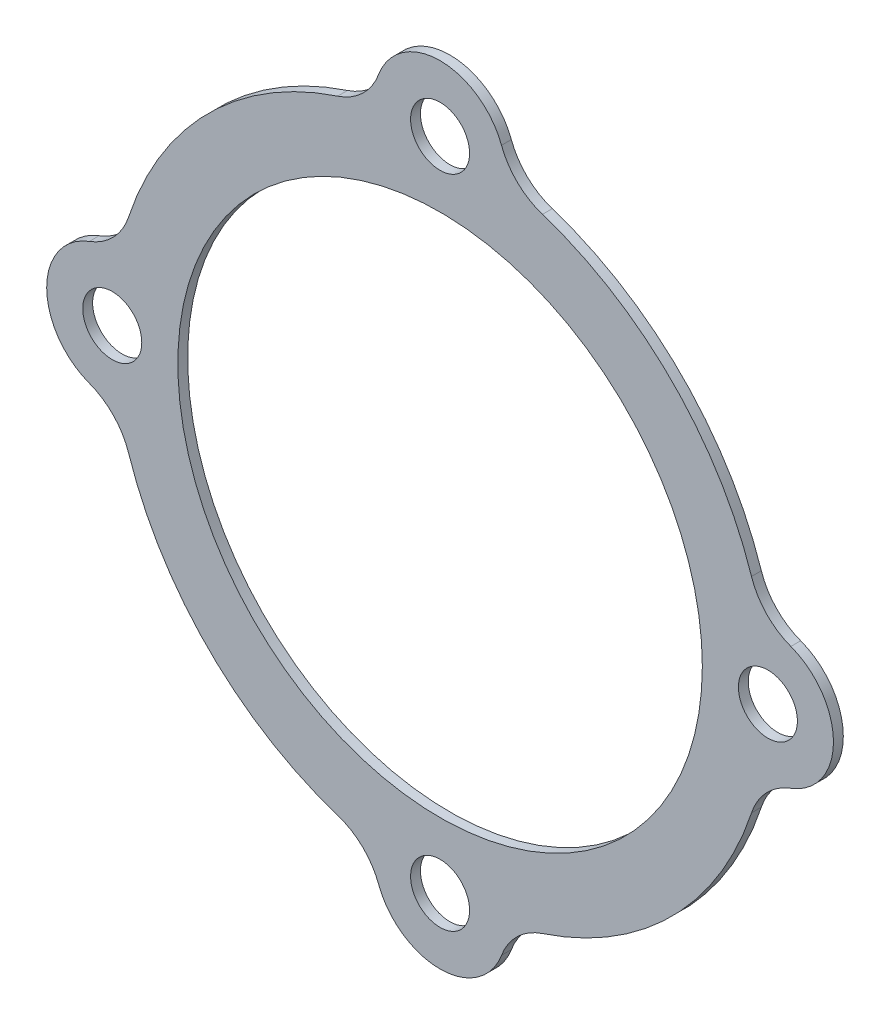
from build123d import *

# Parameters (mm, degrees)
SKETCH_1_R      = 40
SKETCH_1_R_2    = 4.5
EXTRUDE_1_DEPTH = 1.5


with BuildPart() as part:
    # 草图1 → 凸台-拉伸1 (new body)
    with BuildSketch(Plane.XY):
        with BuildLine():
            ThreePointArc((15.612494996, -47.5), (35.355339059, -35.355339059), (47.5, -15.612494996))
            ThreePointArc((47.5, -15.612494996), (49.788897449, -11.806790765), (53.5, -9.367496998))
            ThreePointArc((53.5, -9.367496998), (60, 0), (53.5, 9.367496998))
            ThreePointArc((53.5, 9.367496998), (49.788897449, 11.806790765), (47.5, 15.612494996))
            ThreePointArc((47.5, 15.612494996), (35.355339059, 35.355339059), (15.612494996, 47.5))
            ThreePointArc((15.612494996, 47.5), (11.806790765, 49.788897449), (9.367496998, 53.5))
            ThreePointArc((9.367496998, 53.5), (0, 60), (-9.367496998, 53.5))
            ThreePointArc((-9.367496998, 53.5), (-11.806790765, 49.788897449), (-15.612494996, 47.5))
            ThreePointArc((-15.612494996, 47.5), (-35.355339059, 35.355339059), (-47.5, 15.612494996))
            ThreePointArc((-47.5, 15.612494996), (-49.788897449, 11.806790765), (-53.5, 9.367496998))
            ThreePointArc((-53.5, 9.367496998), (-60, 0), (-53.5, -9.367496998))
            ThreePointArc((-53.5, -9.367496998), (-49.788897449, -11.806790765), (-47.5, -15.612494996))
            ThreePointArc((-47.5, -15.612494996), (-35.355339059, -35.355339059), (-15.612494996, -47.5))
            ThreePointArc((-15.612494996, -47.5), (-11.806790765, -49.788897449), (-9.367496998, -53.5))
            ThreePointArc((-9.367496998, -53.5), (0, -60), (9.367496998, -53.5))
            ThreePointArc((9.367496998, -53.5), (11.806790765, -49.788897449), (15.612494996, -47.5))
        make_face()
        Circle(SKETCH_1_R, mode=Mode.SUBTRACT)
        with Locations((0, 50)):
            Circle(SKETCH_1_R_2, mode=Mode.SUBTRACT)
        with Locations((-50, 0)):
            Circle(SKETCH_1_R_2, mode=Mode.SUBTRACT)
        with Locations((0, -50)):
            Circle(SKETCH_1_R_2, mode=Mode.SUBTRACT)
        with Locations((50, 0)):
            Circle(SKETCH_1_R_2, mode=Mode.SUBTRACT)
    extrude(amount=EXTRUDE_1_DEPTH)


solid = part.part
